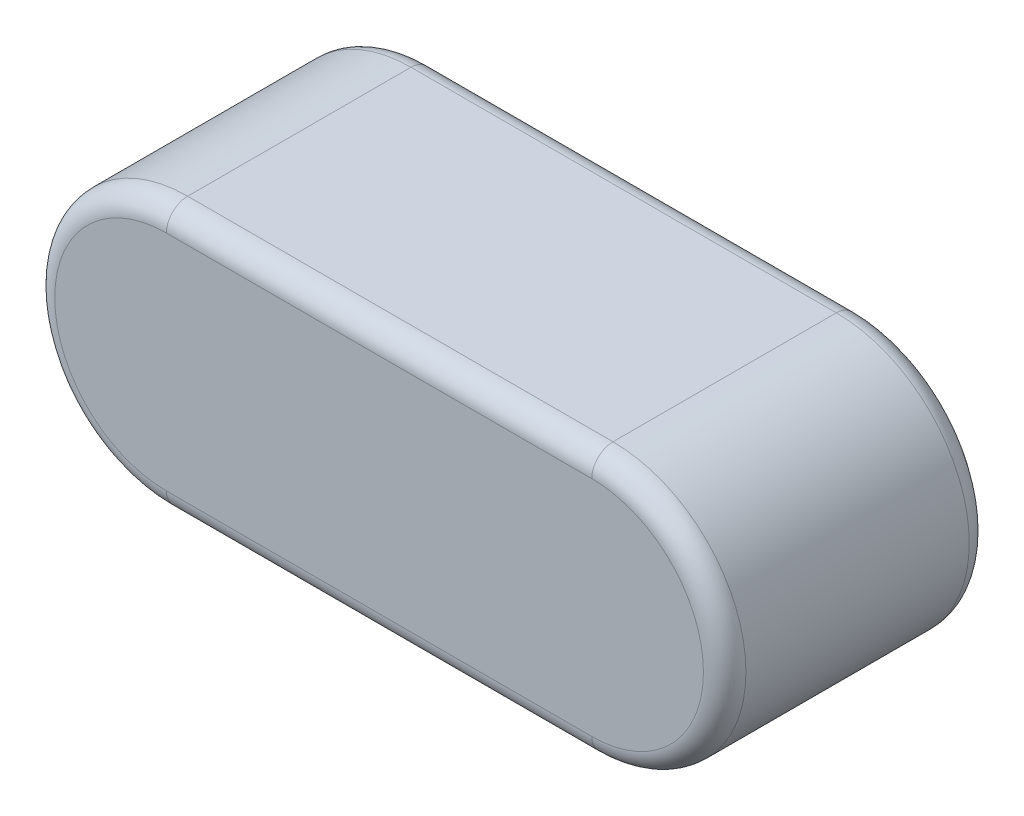
from build123d import *

# Parameters (mm, degrees)
BASE_EXTRUDE_DEPTH = 5
FILLET1_R          = 0.4


with BuildPart() as part:
    # Sketch1 → Base-Extrude (new body)
    with BuildSketch(Plane.XY):
        with BuildLine():
            Line((-4, 2.5), (4, 2.5))
            ThreePointArc((4, 2.5), (6.5, 0), (4, -2.5))
            Line((4, -2.5), (-4, -2.5))
            ThreePointArc((-4, -2.5), (-6.5, 0), (-4, 2.5))
        make_face()
    extrude(amount=BASE_EXTRUDE_DEPTH)

    # Fillet1
    fillet1_edges = [part.edges().sort_by_distance(p)[0] for p in [
        (6.5, 0, 5),
        (0, 2.5, 5),
        (-6.5, 0, 5),
        (0, 2.5, 0),
        (6.5, 0, 0),
        (0, -2.5, 0),
        (-6.5, 0, 0),
        (0, -2.5, 5),
    ]]
    fillet(fillet1_edges, radius=FILLET1_R)


solid = part.part
